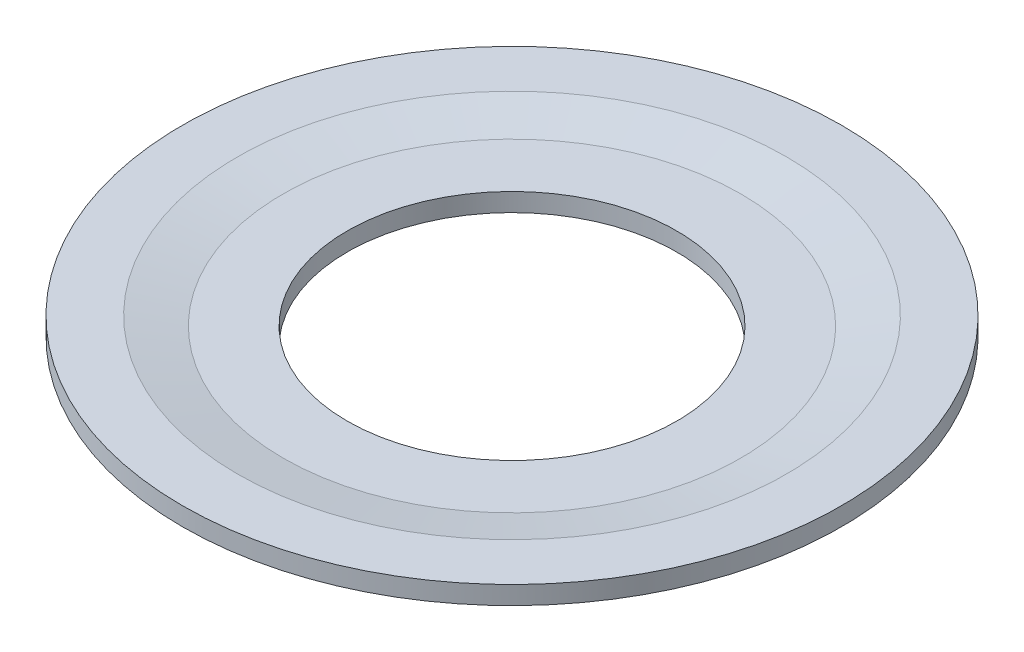
SolidWorks part; units mm, degrees
ref_plane "Front" through (0, 0, 0) normal (0, 0, 1) x (1, 0, 0)
ref_plane "Top" through (0, 0, 0) normal (0, 1, 0) x (1, 0, 0)
ref_plane "Right" through (0, 0, 0) normal (1, 0, 0) x (0, 0, -1)
sketch "Sketch1" plane through (0, 0, 0) normal (0, 0, 1) x (1, 0, 0)
  line L0 (0, 0) -> (0, 2)
  line L1 (0, 2) -> (7, 2)
  line L2 (0, 0) -> (6, 0)
  line L3 (18, 2.9973) -> (18, 1)
  line L4 (18, 2.9973) -> (12, 2.9973)
  line L5 (18, 1) -> (12, 1)
  line L6 (7, 2) -> (12, 2.9973)
  line L7 (6, 0) -> (12, 1)
  line L8 (-18, 6.7767) -> (-18, -5.2031) construction
  dimension "D1" = 2
  dimension "D2" = 7
  dimension "D3" = 18
  dimension "D4" = 6
  dimension "D5" = 2.9973
  dimension "D6" = 6
  dimension "D7" = 1
  dimension "D8" = 18
revolve "Revolve1" add sketch "Sketch1" angle 360 about L8
scale "Scale 1" bodies to scale 102 scale about centroid uniform scaling yes scale factor 1.875
